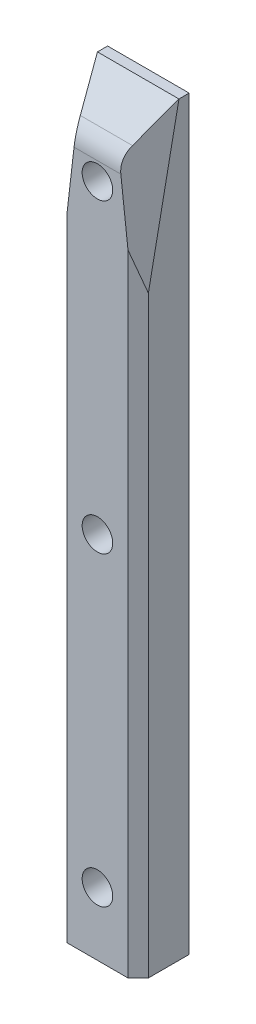
from build123d import *

# Parameters (mm, degrees)
SKETCH1_W                                          = 40
SKETCH1_H                                          = 366
BOSS_EXTRUDE1_DEPTH                                = 25
SKETCH4_R                                          = 7.5
CUT_EXTRUDE1_DEPTH                                 = 2
HOLE_SIZE_BASED_ON_HEX_SOCKET_CAP_SCRE_D           = 9
HOLE_SIZE_BASED_ON_HEX_SOCKET_CAP_SCRE_CBORE_D     = 15
HOLE_SIZE_BASED_ON_HEX_SOCKET_CAP_SCRE_CBORE_DEPTH = 10
CUT_EXTRUDE4_DEPTH                                 = 15
CHAMFER4_SIZE                                      = 5
CUT_EXTRUDE5_DEPTH                                 = 189.981480574
FILLET3_R                                          = 15


with BuildPart() as part:
    # Sketch1 → Boss-Extrude1 (new body)
    with BuildSketch(Plane.XY):
        Rectangle(SKETCH1_W, SKETCH1_H)
    extrude(amount=BOSS_EXTRUDE1_DEPTH)

    # Sketch4 → Cut-Extrude1 (cut)
    with BuildSketch(Plane.XY.offset(25)):
        with Locations((0, -152)):
            Circle(SKETCH4_R)
        with Locations((0, -2)):
            Circle(SKETCH4_R)
        with Locations((0, 148)):
            Circle(SKETCH4_R)
    extrude(amount=-CUT_EXTRUDE1_DEPTH, mode=Mode.SUBTRACT)

    # Hole Size (based on) hex socket cap screw type 1 (through all)
    with Locations(Plane.XY.offset(23)):
        with Locations((0, -152), (0, -2), (0, 148)):
            CounterBoreHole(HOLE_SIZE_BASED_ON_HEX_SOCKET_CAP_SCRE_D / 2, HOLE_SIZE_BASED_ON_HEX_SOCKET_CAP_SCRE_CBORE_D / 2, HOLE_SIZE_BASED_ON_HEX_SOCKET_CAP_SCRE_CBORE_DEPTH)

    # Sketch13 → Cut-Extrude4 (cut)
    with BuildSketch(Plane(origin=(-32.686463761, 3.77430773, 18.871538651), x_dir=(0.46855304860894914, -0.22010109077968257, 0.855577904387937), z_dir=(-0.8617274844321422, 0.09950371902099794, 0.49751859510498975))):
        Polygon((-6.250003897, 80.225632862), (-22.8497284, 179.511998894), (-45.371671063, 174.403630071), align=None)
    cut_extrude4 = extrude(amount=CUT_EXTRUDE4_DEPTH, mode=Mode.SUBTRACT)

    # Mirror1: Cut-Extrude4 across plane
    add(cut_extrude4.mirror(Plane.ZY), mode=Mode.SUBTRACT)

    # Chamfer4
    chamfer4_edges = [part.edges().sort_by_distance(p)[0] for p in [
        (-20, -50, 25),
        (20, -50, 25),
    ]]
    chamfer(chamfer4_edges, length=CHAMFER4_SIZE)

    # Sketch14 → Cut-Extrude5 (cut, through all)
    with BuildSketch(Plane.ZY.offset(20)):
        Polygon((5, 183), (25, 163), (25, 183), align=None)
    extrude(amount=-CUT_EXTRUDE5_DEPTH, mode=Mode.SUBTRACT)

    # Fillet3
    fillet3_edges = [part.edges().sort_by_distance(p)[0] for p in [
        (0, 163, 25),
    ]]
    fillet(fillet3_edges, radius=FILLET3_R)


solid = part.part
